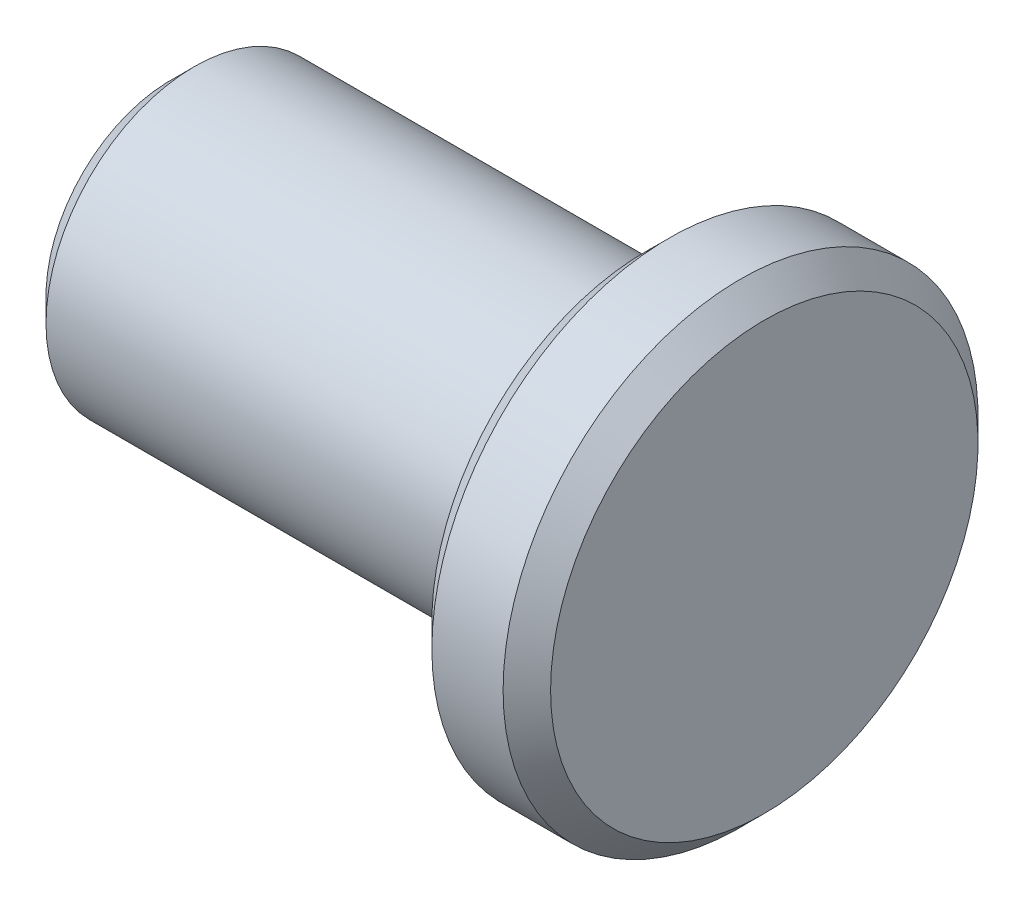
SolidWorks part; units mm, degrees
material "45#"
ref_plane "前视基准面" through (0, 0, 0) normal (0, 0, 1) x (1, 0, 0)
ref_plane "上视基准面" through (0, 0, 0) normal (0, 1, 0) x (1, 0, 0)
ref_plane "右视基准面" through (0, 0, 0) normal (1, 0, 0) x (0, 0, -1)
sketch "草图1" plane through (0, 0, 0) normal (0, 0, 1) x (1, 0, 0)
  line L0 (232.9371, -170.509) -> (256.9371, -170.509) construction
  line L1 (232.9371, -310.509) -> (232.9371, 209.491) construction
  line L3 (236.9371, -170.509) -> (236.9371, -164.259)
  line L4 (244.9371, -164.259) -> (232.9371, -164.259) construction
  line L5 (236.9371, -164.259) -> (256.9371, -164.259)
  line L6 (256.9371, -164.259) -> (256.9371, -160.509)
  line L7 (256.9371, -205.509) -> (256.9371, -147.009) construction
  line L8 (256.9371, -160.509) -> (261.9371, -160.509)
  line L9 (261.9371, -160.509) -> (261.9371, -170.509)
  line L10 (236.9371, -170.509) -> (261.9371, -170.509)
  dimension "D1" = 20
  dimension "D2" = 5
  dimension "D3" = 20
revolve "旋转1" add sketch "草图1" angle 360 about L0
chamfer "倒角1" distance 1 angle 45 3 edges at (261.9371, -170.509, 10) (256.9371, -170.509, 10) (236.9371, -170.509, 6.25)
